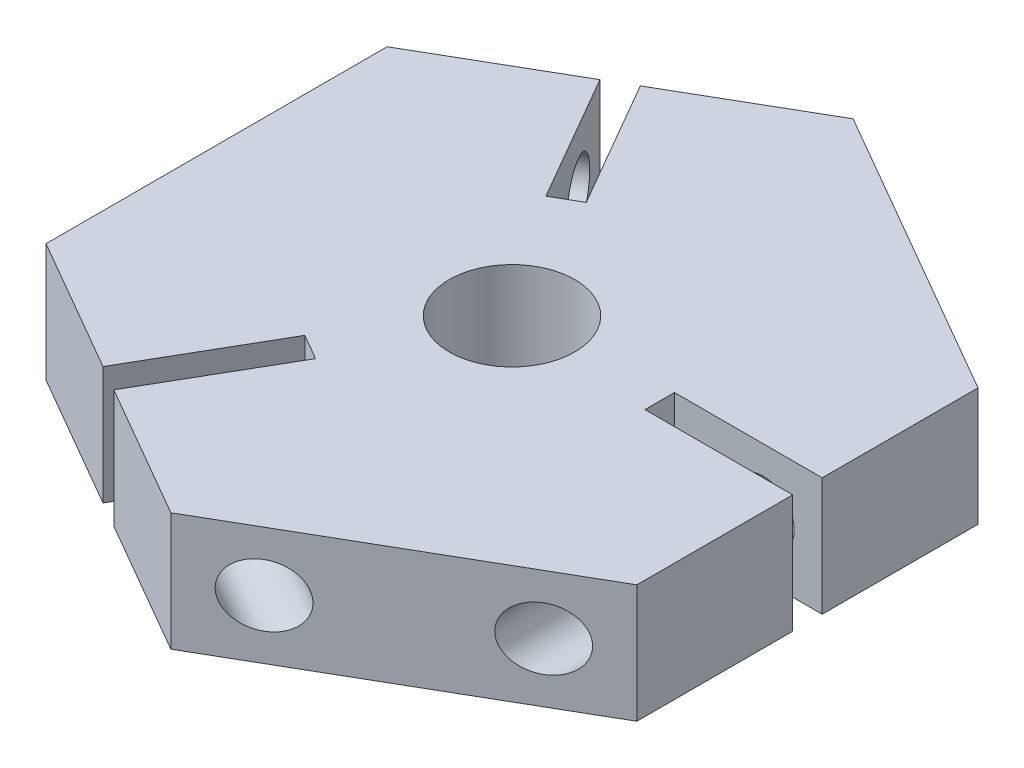
from build123d import *

# Parameters (mm, degrees)
BOSS_EXTRUDE1_DEPTH = 8
SKETCH2_R           = 4.25
CUT_EXTRUDE1_DEPTH  = 10
CUT_EXTRUDE3_DEPTH  = 10
CIRPATTERN1_COUNT   = 3
SKETCH4_R           = 2.1
CUT_EXTRUDE4_DEPTH  = 33.3190556
CIRPATTERN2_COUNT   = 3
SKETCH6_R           = 2.15
CUT_EXTRUDE6_DEPTH  = 10


with BuildPart() as part:
    # Sketch1 → Boss-Extrude1 (new body)
    with BuildSketch(Plane(origin=(0, 0, 0), x_dir=(1, 0, 0), z_dir=(0, 1, 0))):
        Polygon((0, 23.094010768), (-20, 11.547005384), (-20, -11.547005384), (0, -23.094010768), (20, -11.547005384), (20, 11.547005384), align=None)
    extrude(amount=BOSS_EXTRUDE1_DEPTH)

    # Sketch2 → Cut-Extrude1 (cut)
    with BuildSketch(Plane(origin=(0, 8, 0), x_dir=(1, 0, 0), z_dir=(0, 1, 0))):
        with Locations(Location((0, 0, 0), (0, 0, 270))):
            Circle(SKETCH2_R)
    extrude(amount=-CUT_EXTRUDE1_DEPTH, mode=Mode.SUBTRACT)

    # Sketch3 → Cut-Extrude3 (cut)
    with BuildSketch(Plane(origin=(0, 8, 0), x_dir=(1, 0, 0), z_dir=(0, 1, 0))):
        Polygon((-9.133974596, 17.820508076), (-10.866025404, 16.820508076), (-5.866025404, 8.160254038), (-4.133974596, 9.160254038), align=None)
    cut_extrude3 = extrude(amount=-CUT_EXTRUDE3_DEPTH, mode=Mode.SUBTRACT)

    # CirPattern1: Cut-Extrude3 ×3 about axis
    cirpattern1_axis = Axis((0, 0, 0), (0, 1, 0))
    for i in range(1, CIRPATTERN1_COUNT):
        add(cut_extrude3.rotate(cirpattern1_axis, i * 360 / CIRPATTERN1_COUNT), mode=Mode.SUBTRACT)

    # Sketch4 → Cut-Extrude4 (cut, symmetric)
    with BuildSketch(Plane.XY.offset(-1)):
        with Locations((16, 4)):
            Circle(SKETCH4_R)
    cut_extrude4 = extrude(amount=CUT_EXTRUDE4_DEPTH, both=True, mode=Mode.SUBTRACT)

    # CirPattern2: Cut-Extrude4 ×3 about axis
    cirpattern2_axis = Axis((0, -2, 0), (0, 1, 0))
    for i in range(1, CIRPATTERN2_COUNT):
        add(cut_extrude4.rotate(cirpattern2_axis, i * 360 / CIRPATTERN2_COUNT), mode=Mode.SUBTRACT)

    # Sketch6 → Cut-Extrude6 (cut)
    with BuildSketch(Plane(origin=(-14.906511483, 7, 5.40190095), x_dir=(1, 0, 0), z_dir=(0, 1, 0))):
        with Locations((10.906511483, 12.330104181)):
            Circle(SKETCH6_R)
        with Locations(Location((18.906511483, -1.52630228, 0), (0, 0, 270))):
            Circle(SKETCH6_R)
    extrude(amount=-CUT_EXTRUDE6_DEPTH, mode=Mode.SUBTRACT)


solid = part.part
